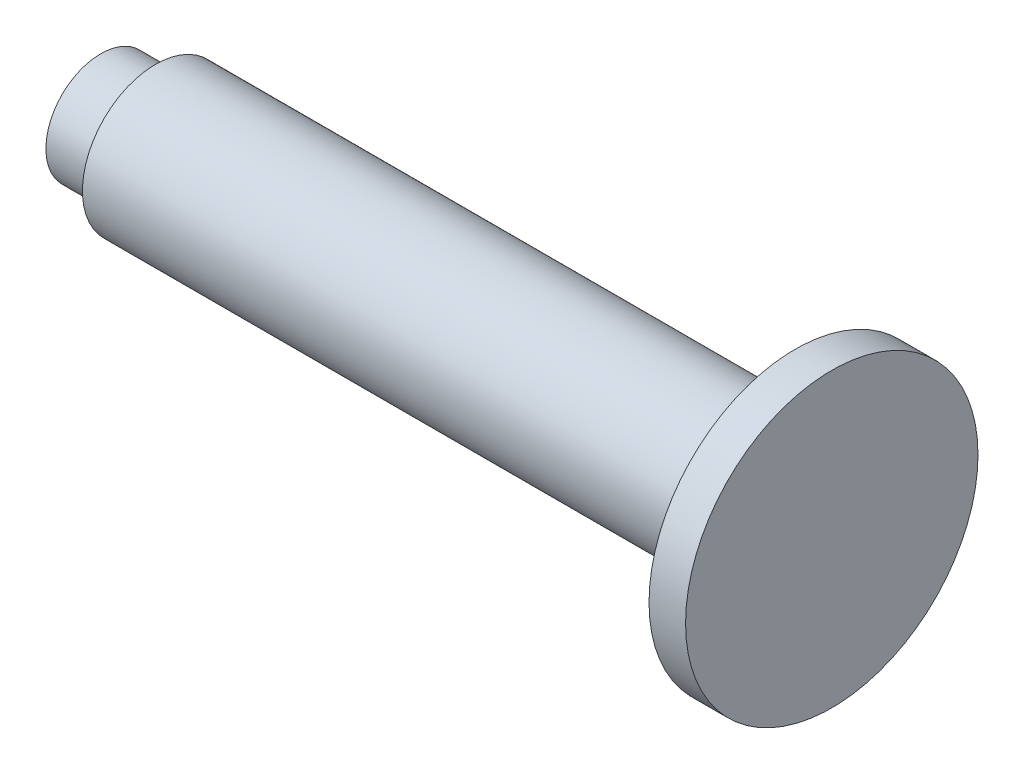
SolidWorks part; units mm, degrees
ref_plane "Front Plane" through (0, 0, 0) normal (0, 0, 1) x (1, 0, 0)
ref_plane "Top Plane" through (0, 0, 0) normal (0, 1, 0) x (1, 0, 0)
ref_plane "Right Plane" through (0, 0, 0) normal (1, 0, 0) x (0, 0, -1)
sketch "Sketch1" plane through (0, 0, 0) normal (0, 0, 1) x (1, 0, 0)
  line L0 (0, 0) -> (0, 3)
  line L1 (0, 3) -> (3, 3)
  line L2 (3, 3) -> (3, 4)
  line L3 (3, 4) -> (38, 4)
  line L4 (38, 4) -> (38, 8)
  line L5 (38, 8) -> (40, 8)
  line L6 (40, 8) -> (40, 0)
  line L7 (40, 0) -> (0, 0)
  dimension "D1" = 8
  dimension "D2" = 2
  dimension "D3" = 35
  dimension "D4" = 3
  dimension "D5" = 4
  dimension "D6" = 3
revolve "Revolve1" add sketch "Sketch1" angle 360 about L7
